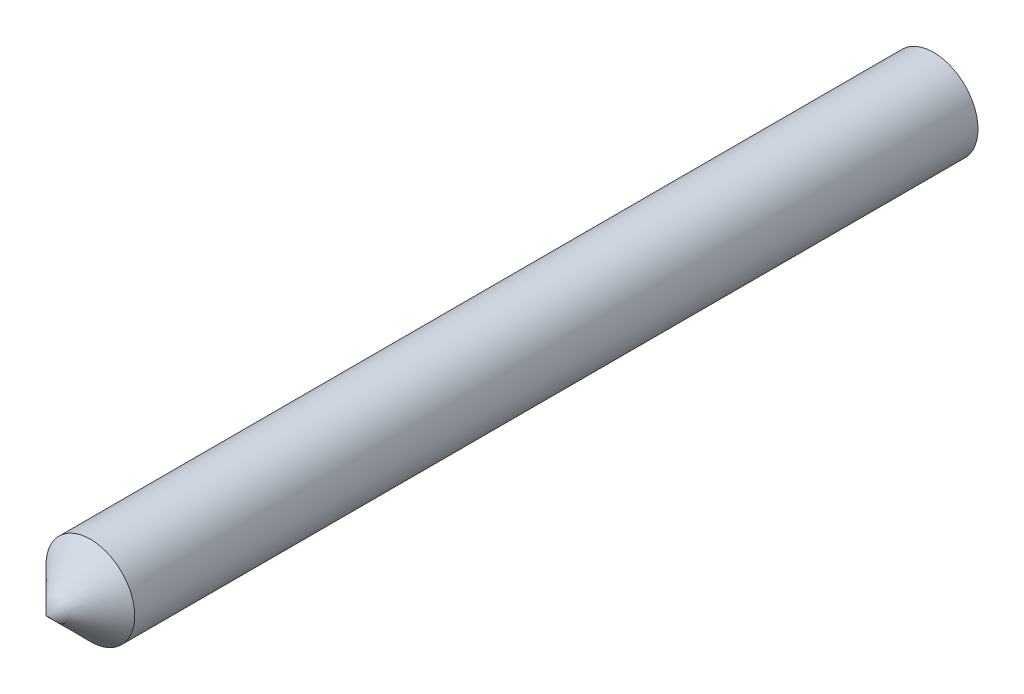
SolidWorks part; units mm, degrees
material "PBT general purpose"
ref_plane "Front Plane" through (0, 0, 0) normal (0, 0, 1) x (1, 0, 0)
ref_plane "Top Plane" through (0, 0, 0) normal (0, 1, 0) x (1, 0, 0)
ref_plane "Right Plane" through (0, 0, 0) normal (1, 0, 0) x (0, 0, -1)
sketch "Sketch1" plane through (0, 0, 0) normal (0, 0, 1) x (1, 0, 0)
  circle A0 centre (0, 0) radius 5
extrude "Boss-Extrude1" add sketch "Sketch1" along normal blind 100
chamfer "Chamfer2" distance 5 angle 45 1 edges at (5, 0, 100)
